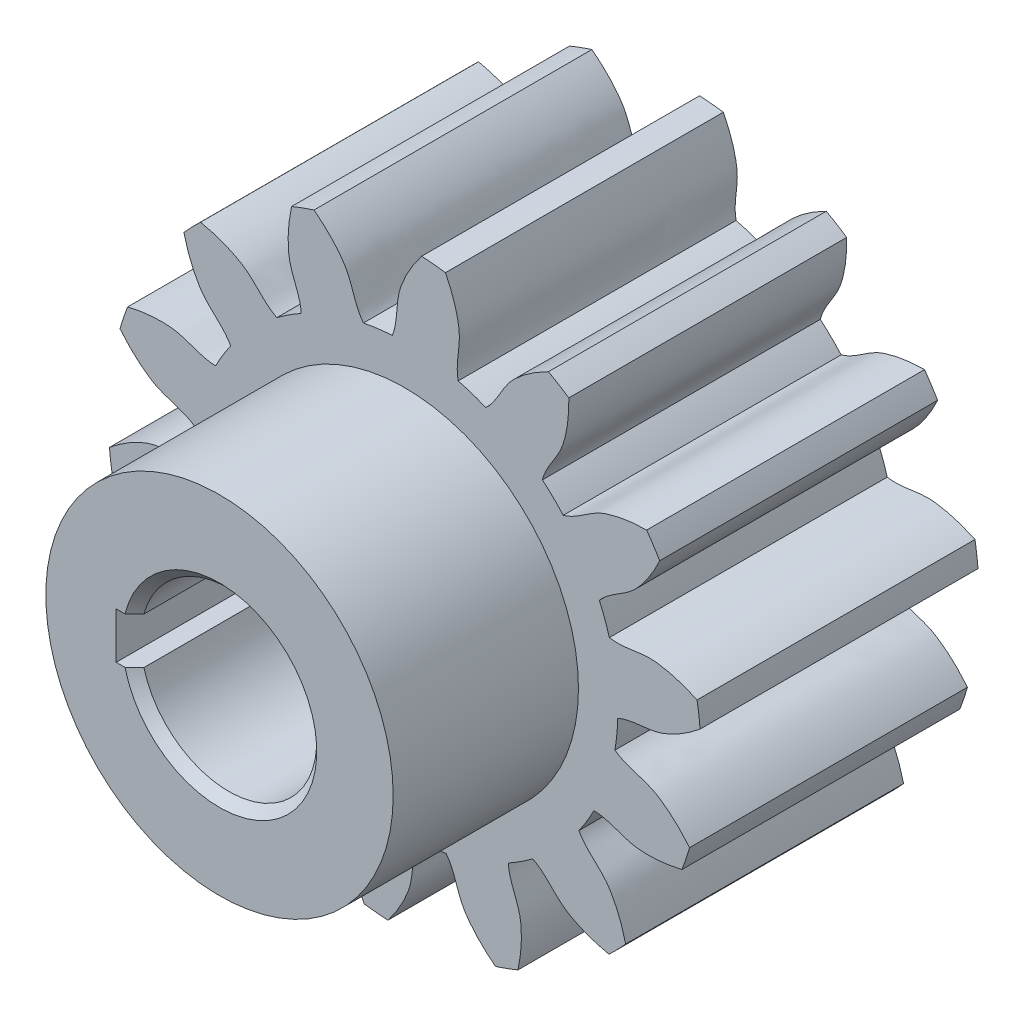
from build123d import *

# Parameters (mm, degrees)
SKETCH1_R           = 46
SKETCH1_R_2         = 19
BOSS_EXTRUDE1_DEPTH = 60
BOSS_EXTRUDE2_DEPTH = 60
CIRPATTERN1_COUNT   = 14
SKETCH3_R           = 37.5
SKETCH3_R_2         = 19
BOSS_EXTRUDE3_DEPTH = 40
SKETCH4_R           = 27.5
CUT_EXTRUDE1_DEPTH  = 22
CHAMFER1_SIZE       = 2
CUT_EXTRUDE2_REACH  = 136.715
SKETCH5_W           = 6.6
SKETCH5_H           = 10


with BuildPart() as part:
    # Sketch1 → Boss-Extrude1 (new body)
    with BuildSketch(Plane.XY):
        Circle(SKETCH1_R)
        Circle(SKETCH1_R_2, mode=Mode.SUBTRACT)
    extrude(amount=BOSS_EXTRUDE1_DEPTH)

    # Sketch2 → Boss-Extrude2 (add)
    with BuildSketch(Plane.XY):
        with BuildLine():
            ThreePointArc((63.104532635, 10.668550086), (63.483720976, 8.112778259), (63.759442112, 5.543784043))
            add(Edge.make_bspline(
                [(63.759442112, 5.543784043), (62.389318996, 4.412517104), (60.251221393, 2.874111803), (57.206354902, 1.300494321), (52.845151495, -0.465750744), (48.767643844, -0.044762334), (45.980655038, -1.333927402)],
                knots=[0, 0, 0, 0, 0.275474679, 0.405578262, 0.530573806, 1, 1, 1, 1], degree=3))
            ThreePointArc((45.980655038, -1.333927402), (45.628924451, 5.831059374), (44.167506403, 12.854235805))
            add(Edge.make_bspline(
                [(63.104532635, 10.668550086), (61.493951486, 11.418903738), (59.037689651, 12.370181839), (55.694944892, 13.127507004), (51.029724893, 13.740237902), (47.189127109, 12.307370657), (44.167506403, 12.854235805)],
                knots=[0, 0, 0, 0, 0.275474679, 0.405578262, 0.530573806, 1, 1, 1, 1], degree=3))
        make_face()
    boss_extrude2 = extrude(amount=BOSS_EXTRUDE2_DEPTH)

    # CirPattern1: Boss-Extrude2 ×14 about axis
    cirpattern1_axis = Axis((0, 0, 60), (0, 0, -1))
    for i in range(1, CIRPATTERN1_COUNT):
        add(boss_extrude2.rotate(cirpattern1_axis, i * 360 / CIRPATTERN1_COUNT))

    # Sketch3 → Boss-Extrude3 (add)
    with BuildSketch(Plane.XY.offset(60)):
        Circle(SKETCH3_R)
        Circle(SKETCH3_R_2, mode=Mode.SUBTRACT)
    extrude(amount=BOSS_EXTRUDE3_DEPTH)

    # Sketch4 → Cut-Extrude1 (cut)
    with BuildSketch(Plane(origin=(0, 0, 0), x_dir=(-1, 0, 0), z_dir=(0, 0, -1))):
        Circle(SKETCH4_R)
    extrude(amount=-CUT_EXTRUDE1_DEPTH, mode=Mode.SUBTRACT)

    # Chamfer1
    chamfer1_edges = [part.edges().sort_by_distance(p)[0] for p in [
        (-19, 0, 100),
    ]]
    chamfer(chamfer1_edges, length=CHAMFER1_SIZE)

    # Sketch5 → Cut-Extrude2 (cut, up to next)
    with BuildSketch(Plane.XY.offset(100), mode=Mode.PRIVATE) as cut_extrude2_sk1:
        with Locations((-19, 0)):
            Rectangle(SKETCH5_W, SKETCH5_H)
    cut_extrude2_tool1 = extrude(cut_extrude2_sk1.sketch, amount=-CUT_EXTRUDE2_REACH, mode=Mode.PRIVATE) & part.part
    add(cut_extrude2_tool1.solids().sort_by_distance((-19, 0, 100))[0], mode=Mode.SUBTRACT)


solid = part.part
